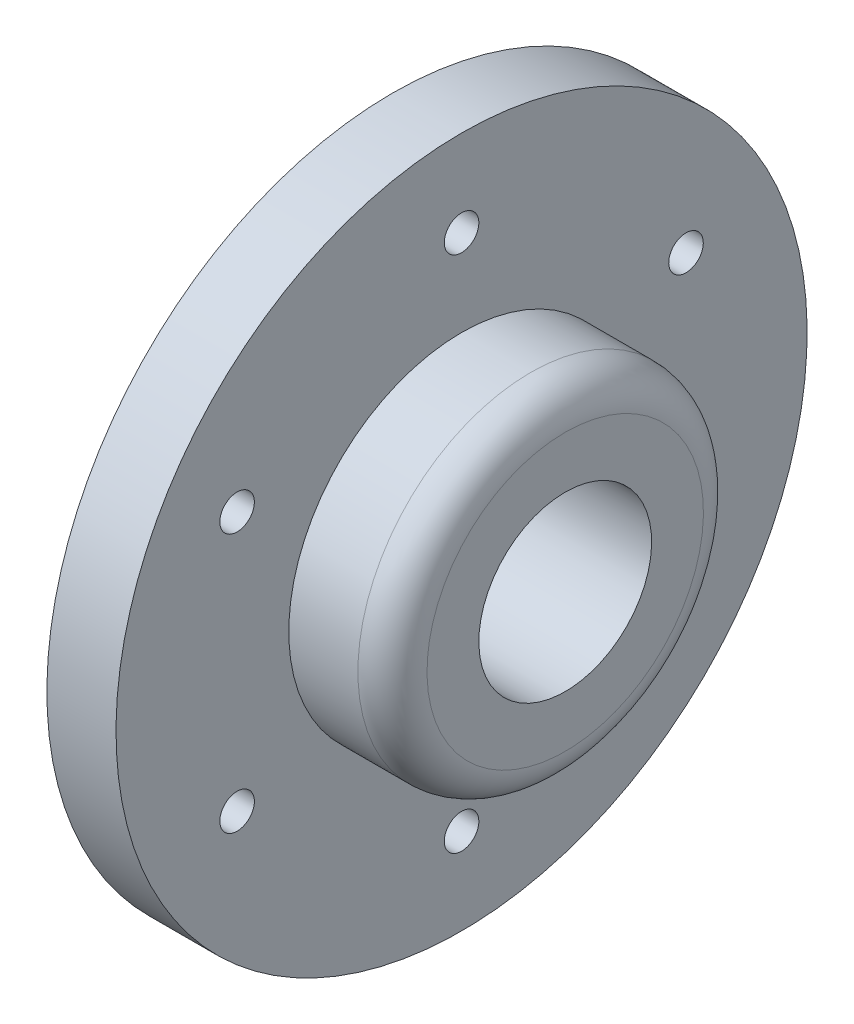
SolidWorks part; units mm, degrees
material "普通碳钢"
ref_plane "Front Plane" through (0, 0, 0) normal (0, 0, 1) x (1, 0, 0)
ref_plane "Top Plane" through (0, 0, 0) normal (0, 1, 0) x (1, 0, 0)
ref_plane "Right Plane" through (0, 0, 0) normal (1, 0, 0) x (0, 0, -1)
sketch "Sketch1" plane through (0, 0, 0) normal (0, 0, 1) x (1, 0, 0)
  line L0 (0, 25) -> (0, 100)
  line L1 (0, 100) -> (20, 100)
  line L2 (20, 100) -> (20, 50)
  line L3 (20, 50) -> (50, 50)
  line L4 (50, 50) -> (50, 25)
  line L5 (113.2139, 0) -> (0, 0) construction
  line L6 (50, 25) -> (0, 25)
  dimension "D1" = 100
  dimension "D2" = 50
  dimension "D3" = 20
  dimension "D4" = 25
  dimension "D5" = 50
revolve "Revolve1" add sketch "Sketch1" angle 360 about L5
sketch "Sketch3" plane through (20, 0, 0) normal (1, 0, 0) x (0, 0, -1)
  line L0 (0, 0) -> (0, 91.9676) construction
  circle A1 centre (0, 75) radius 5
  dimension "D1" = 75
  dimension "D2" = 10
extrude "Cut-Extrude1" cut sketch "Sketch3" against normal up to next
pattern_circular "CirPattern1" count 6 over 360 about axis through (0, 0, 0) along (1, 0, 0) of "Cut-Extrude1"
fillet "Fillet1" radius 10 1 edges at (50, 50, 0)
